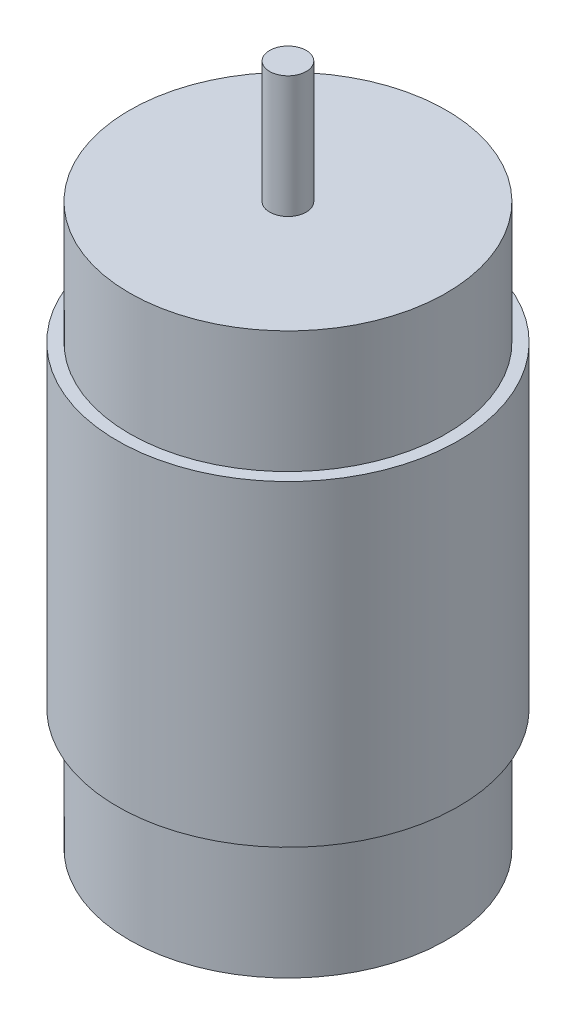
from build123d import *

# Parameters (mm, degrees)
SKETCH1_R           = 13
BOSS_EXTRUDE1_DEPTH = 10
SKETCH2_R           = 14
BOSS_EXTRUDE2_DEPTH = 26
SKETCH3_R           = 13
BOSS_EXTRUDE3_DEPTH = 10
SKETCH4_R           = 1.5
BOSS_EXTRUDE4_DEPTH = 10


with BuildPart() as part:
    # Sketch1 → Boss-Extrude1 (new body)
    with BuildSketch(Plane(origin=(0, 0, 0), x_dir=(1, 0, 0), z_dir=(0, 1, 0))):
        with Locations(Location((0, 0, 0), (0, 0, 270))):
            Circle(SKETCH1_R)
    extrude(amount=BOSS_EXTRUDE1_DEPTH)

    # Sketch2 → Boss-Extrude2 (add)
    with BuildSketch(Plane(origin=(0, 10, 0), x_dir=(1, 0, 0), z_dir=(0, 1, 0))):
        with Locations(Location((0, 0, 0), (0, 0, 90))):
            Circle(SKETCH2_R)
    extrude(amount=BOSS_EXTRUDE2_DEPTH)

    # Sketch3 → Boss-Extrude3 (add)
    with BuildSketch(Plane(origin=(0, 36, 0), x_dir=(1, 0, 0), z_dir=(0, 1, 0))):
        with Locations(Location((0, 0, 0), (0, 0, 270))):
            Circle(SKETCH3_R)
    extrude(amount=BOSS_EXTRUDE3_DEPTH)

    # Sketch4 → Boss-Extrude4 (add)
    with BuildSketch(Plane(origin=(0, 46, 0), x_dir=(1, 0, 0), z_dir=(0, 1, 0))):
        with Locations(Location((0, 0, 0), (0, 0, 270))):
            Circle(SKETCH4_R)
    extrude(amount=BOSS_EXTRUDE4_DEPTH)


solid = part.part
